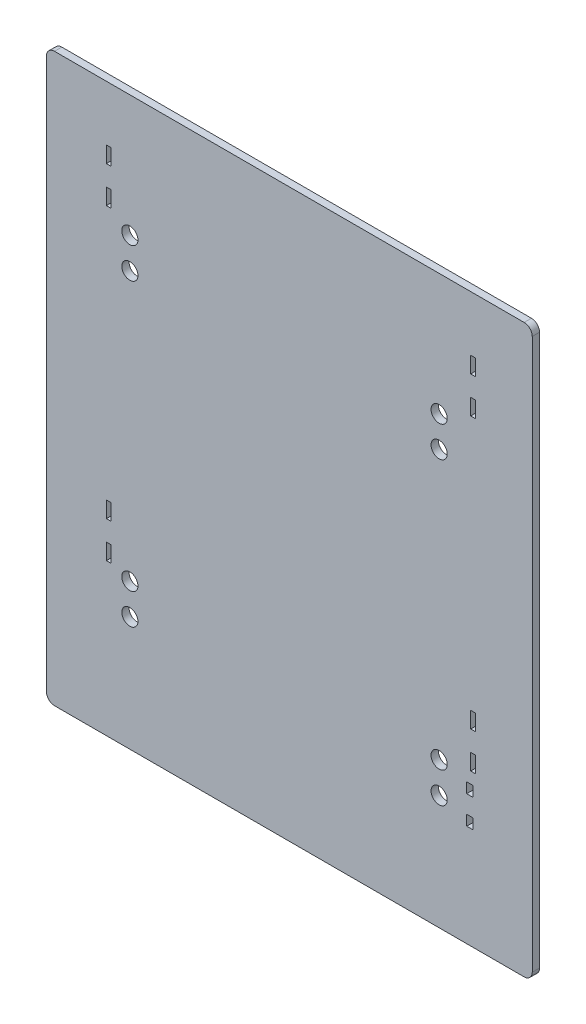
from build123d import *

# Parameters (mm, degrees)
SKETCH1_W                   = 600
SKETCH1_H                   = 700
BOSS_EXTRUDE1_DEPTH         = 9
FILLET1_R                   = 10
SKETCH3_R                   = 10
CUT_EXTRUDE2_DEPTH          = 41
SKETCH7_W                   = 8
SKETCH7_H                   = 12.747725193
CUT_EXTRUDE4_DEPTH          = 483.221865906
CUT_EXTRUDE8_START          = -499.177752008
SKETCH11_W                  = 6
SKETCH11_H                  = 19.989610894
SKETCH11_H_2                = 19.927609768
CUT_EXTRUDE8_DEPTH          = 881.951690015
LPATTERN4_COUNT             = 2
LPATTERN4_PITCH             = 379.75
LPATTERN5_COUNT             = 2
LPATTERN5_PITCH             = 450
LPATTERN5_START             = -499.177752008
LPATTERN5_COPY_1_SKETCH_W   = 6
LPATTERN5_COPY_1_SKETCH_H   = 19.989610894
LPATTERN5_COPY_1_SKETCH_H_2 = 19.927609768
LPATTERN5_COPY_1_DEPTH      = 881.951690015


with BuildPart() as part:
    # Sketch1 → Boss-Extrude1 (new body)
    with BuildSketch(Plane.XY):
        Rectangle(SKETCH1_W, SKETCH1_H)
    extrude(amount=BOSS_EXTRUDE1_DEPTH)

    # Fillet1
    fillet1_edges = [part.edges().sort_by_distance(p)[0] for p in [
        (300, -350, 4.5),
        (-300, -350, 4.5),
        (-300, 350, 4.5),
        (300, 350, 4.5),
    ]]
    fillet(fillet1_edges, radius=FILLET1_R)

    # Sketch3 → Cut-Extrude2 (cut)
    with BuildSketch(Plane(origin=(-23.01798078, 7.933390522, 0), x_dir=(-1, 0, 0), z_dir=(0, 0, -1))):
        with Locations((-208.01798078, 153.666609478)):
            Circle(SKETCH3_R)
        with Locations((-208.01798078, -216.333390522)):
            Circle(SKETCH3_R)
        with Locations((-208.01798078, -178.233390522)):
            Circle(SKETCH3_R)
        with Locations((173.98201922, 191.766609478)):
            Circle(SKETCH3_R)
        with Locations((173.98201922, 153.666609478)):
            Circle(SKETCH3_R)
        with Locations((173.98201922, -178.233390522)):
            Circle(SKETCH3_R)
        with Locations((173.98201922, -216.333390522)):
            Circle(SKETCH3_R)
        with Locations((-208.01798078, 191.766609478)):
            Circle(SKETCH3_R)
    extrude(amount=-CUT_EXTRUDE2_DEPTH, mode=Mode.SUBTRACT)

    # Sketch7 → Cut-Extrude4 (cut, through all)
    with BuildSketch(Plane(origin=(-23.01798078, 7.933390522, 0), x_dir=(-1, 0, 0), z_dir=(0, 0, -1))):
        with Locations((-246.01798078, -191.1057938)):
            Rectangle(SKETCH7_W, SKETCH7_H)
        with Locations((-246.01798078, -225.853518993)):
            Rectangle(SKETCH7_W, SKETCH7_H)
    extrude(amount=-CUT_EXTRUDE4_DEPTH, mode=Mode.SUBTRACT)

    # Sketch11 → Cut-Extrude8 (cut)
    with BuildSketch(Plane(origin=(-23.01798078, 7.93041319, -116.40444969), x_dir=(-1, 0, 0), z_dir=(1.1016286228319074e-14, -8.013698647454937e-05, -0.9999999967890317)).offset(CUT_EXTRUDE8_START)):
        with Locations((199.98201922, -115.795126315)):
            Rectangle(SKETCH11_W, SKETCH11_H)
        with Locations((199.98201922, -160.770464654)):
            Rectangle(SKETCH11_W, SKETCH11_H_2)
    cut_extrude8 = extrude(amount=CUT_EXTRUDE8_DEPTH, mode=Mode.SUBTRACT)

    # LPattern4: Cut-Extrude8 ×2
    with Locations(*[Vector(0, 0.9999999967890317, -8.013698647454937e-05) * (i * LPATTERN4_PITCH) for i in range(1, LPATTERN4_COUNT)]):
        add(cut_extrude8, mode=Mode.SUBTRACT)

    # LPattern5: Cut-Extrude8 ×2
    with Locations(*[(i * LPATTERN5_PITCH, 0, 0) for i in range(1, LPATTERN5_COUNT)]):
        add(cut_extrude8, mode=Mode.SUBTRACT)

    # LPattern5 copy 1 sketch → LPattern5 copy 1 (cut)
    with BuildSketch(Plane(origin=(426.98201922, 387.680411971, -116.434881711), x_dir=(-1, 0, 0), z_dir=(1.1016286228319074e-14, -8.013698647454937e-05, -0.9999999967890317)).offset(LPATTERN5_START)):
        with Locations((199.98201922, -115.795126315)):
            Rectangle(LPATTERN5_COPY_1_SKETCH_W, LPATTERN5_COPY_1_SKETCH_H)
        with Locations((199.98201922, -160.770464654)):
            Rectangle(LPATTERN5_COPY_1_SKETCH_W, LPATTERN5_COPY_1_SKETCH_H_2)
    extrude(amount=LPATTERN5_COPY_1_DEPTH, mode=Mode.SUBTRACT)


solid = part.part
